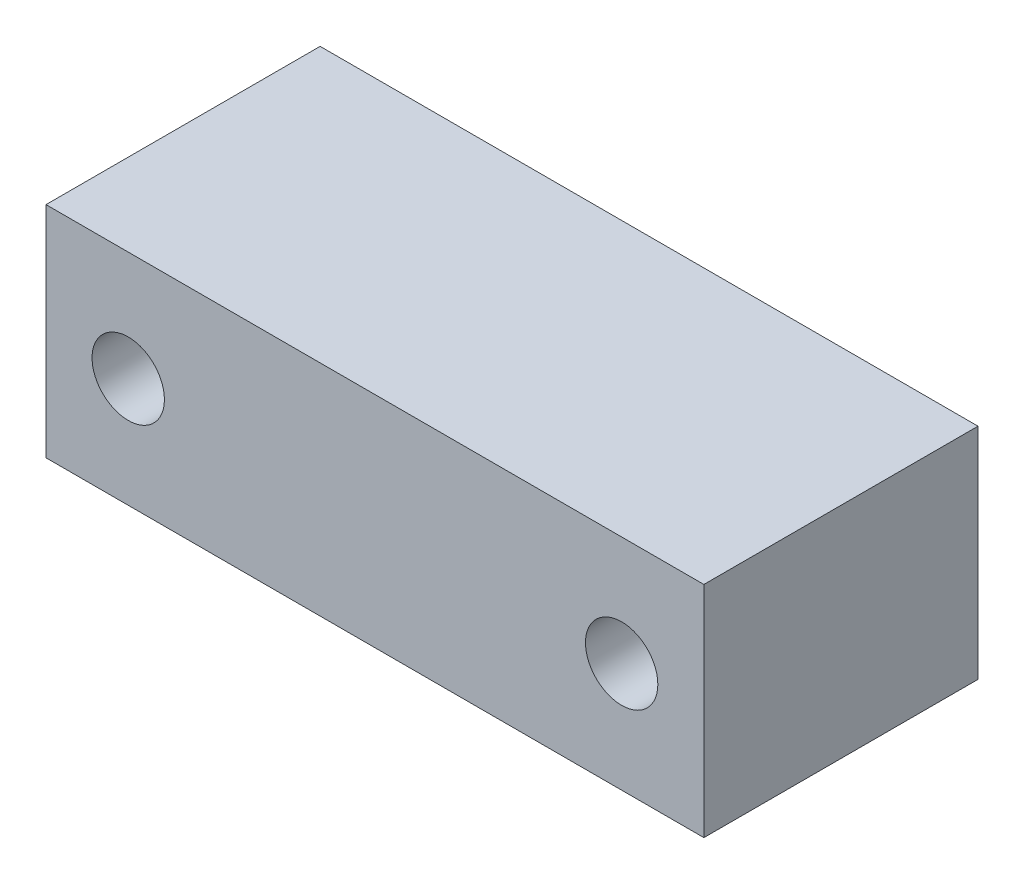
SolidWorks part; units mm, degrees
ref_plane "前视基准面" through (0, 0, 0) normal (0, 0, 1) x (1, 0, 0)
ref_plane "上视基准面" through (0, 0, 0) normal (0, 1, 0) x (1, 0, 0)
ref_plane "右视基准面" through (0, 0, 0) normal (1, 0, 0) x (0, 0, -1)
sketch "草图1" plane through (0, 0, 0) normal (0, 0, 1) x (1, 0, 0)
  line L1 (30, -10) -> (-30, -10)
  line L2 (30, -10) -> (30, 10)
  line L3 (30, 10) -> (-30, 10)
  line L4 (-30, -10) -> (-30, 10)
  line L5 (30, -10) -> (-30, 10) construction
  line L6 (30, 10) -> (-30, -10) construction
  point P0 (0, 0)
  dimension "D1" = 60
  dimension "D2" = 20
extrude "凸台-拉伸1" add sketch "草图1" along normal blind 25
hole_wizard "M6 间隙孔1" positions "草图4" profile "草图3" hole size "M6" standard "GB" end condition up to next
sketch "草图4" plane through (0, 0, 25) normal (0, 0, 1) x (1, 0, 0)
  line L0 (-22.5, 0) -> (0, 0) construction
  line L1 (0, 0) -> (0, 7.4261) construction
  point P0 (-22.5, 0)
  point P2 (22.5, 0)
  point P11 (0, 0)
  point P12 (0, 0)
  dimension "D1" = 45
sketch "草图3" plane through (-22.5, 0, 25) normal (1, 0, 0) x (0, -1, 0)
  line L0 (0, 0) -> (0, 25)
  line L1 (0, 25) -> (3.3, 25)
  line L2 (3.3, 25) -> (3.3, 0)
  line L5 (3.3, 0) -> (0, 0)
  line L11 (0, -6.35) -> (0, 107.95) construction
  dimension "通孔孔直径" = 6.6
  dimension "通孔孔深度" = 25
